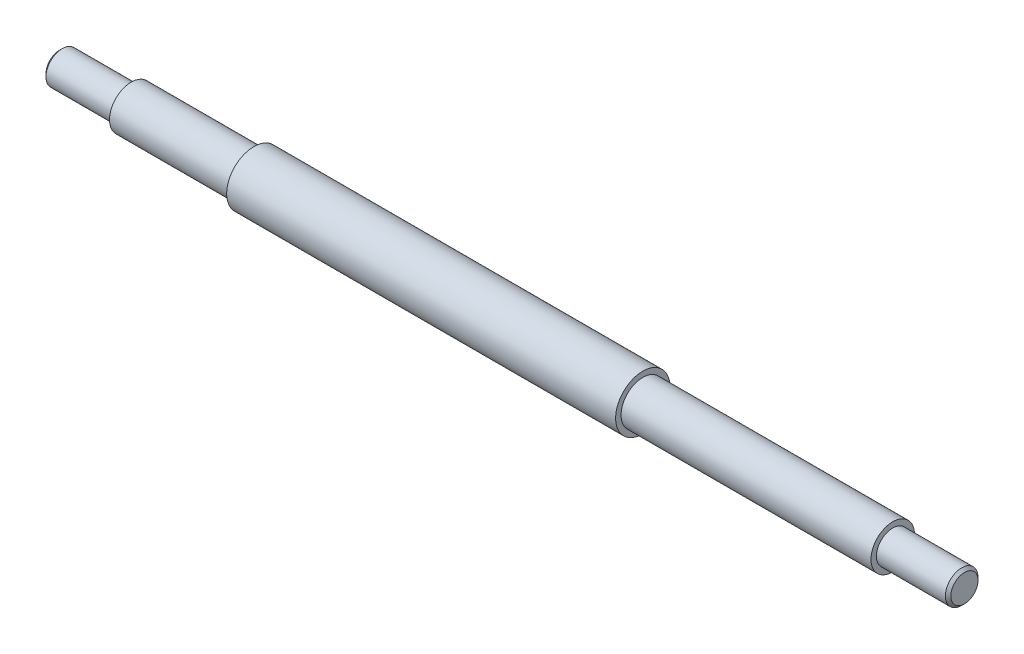
SolidWorks part; units mm, degrees
ref_plane "Front Plane" through (0, 0, 0) normal (0, 0, 1) x (1, 0, 0)
ref_plane "Top Plane" through (0, 0, 0) normal (0, 1, 0) x (1, 0, 0)
ref_plane "Right Plane" through (0, 0, 0) normal (1, 0, 0) x (0, 0, -1)
sketch "Model" plane through (0, 0, 0) normal (0, 0, 1) x (1, 0, 0)
  line L0 (-193.0717, -28.2054) -> (-193.0717, -27.2054)
  line L1 (-53.0717, -28.2054) -> (-53.0717, -27.2054)
  line L2 (-193.0717, -28.2054) -> (-199.0717, -28.2054)
  line L3 (-53.0717, -28.2054) -> (-41.6717, -28.2054)
  line L4 (-206.2485, -28.7054) -> (-206.2485, -31.2054)
  line L5 (-199.0717, -28.2054) -> (-205.7485, -28.2054)
  line L6 (-206.2485, -28.7054) -> (-205.7485, -28.2054)
  line L7 (-39.895, -28.7054) -> (-39.895, -31.2054)
  line L8 (-41.6717, -28.2054) -> (-40.395, -28.2054)
  line L9 (-39.895, -28.7054) -> (-40.395, -28.2054)
  line L11 (-170.5266, -27.2054) -> (-170.5266, -26.2054)
  line L12 (-99.0224, -26.2054) -> (-99.0224, -27.2054)
  line L13 (-170.5266, -26.2054) -> (-99.0224, -26.2054)
  line L14 (-53.0717, -27.2054) -> (-99.0224, -27.2054)
  line L15 (-170.5266, -27.2054) -> (-193.0717, -27.2054)
  line L17 (-206.2485, -31.2054) -> (-228.0859, -31.2054) construction
  line L18 (-206.2485, -31.2054) -> (-39.895, -31.2054)
revolve "Revolve1" add sketch "Model" angle 360 about L17
